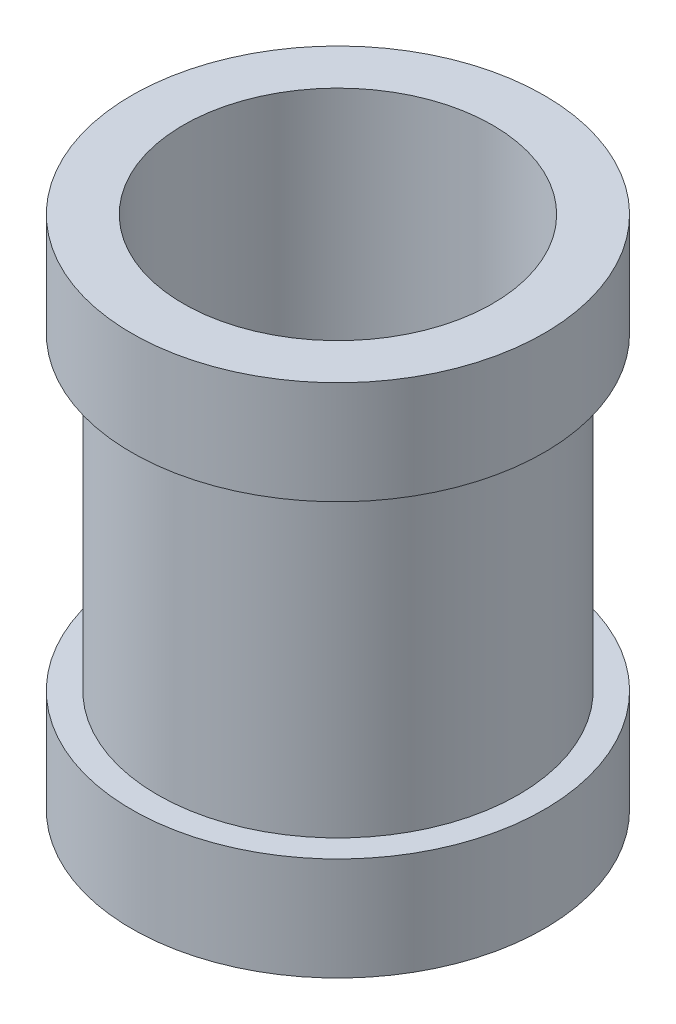
SolidWorks part; units mm, degrees
material "2.0321 (CuZn37)"
ref_plane "Front" through (0, 0, 0) normal (0, 0, 1) x (1, 0, 0)
ref_plane "Top" through (0, 0, 0) normal (0, 1, 0) x (1, 0, 0)
ref_plane "Right" through (0, 0, 0) normal (1, 0, 0) x (0, 0, -1)
sketch "Sketch1" plane through (0, 0, 0) normal (0, 0, 1) x (1, 0, 0)
  line L0 (0, 0) -> (0, 5) construction
  line L1 (1.5, 0) -> (2, 0)
  line L2 (2, 0) -> (2, 1)
  line L3 (2, 1) -> (1.75, 1)
  line L4 (1.75, 1) -> (1.75, 4)
  line L5 (1.75, 4) -> (2, 4)
  line L6 (2, 4) -> (2, 5)
  line L7 (2, 5) -> (1.5, 5)
  line L8 (1.5, 5) -> (1.5, 0)
  dimension "D1" = 5
  dimension "D2" = 1.5
  dimension "D3" = 1.75
  dimension "D4" = 2
  dimension "D5" = 1
revolve "Revolve1" add sketch "Sketch1" angle 360 about L0
